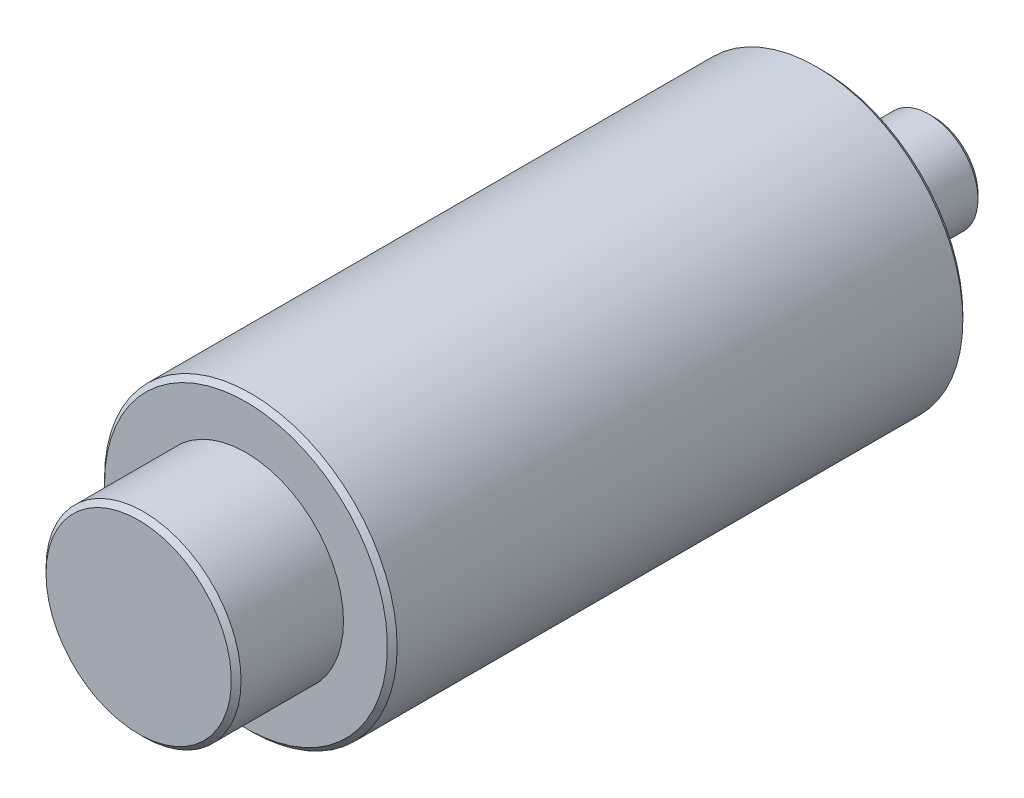
from build123d import *

# Parameters (mm, degrees)
CHAMFER1_SIZE = 0.5


with BuildPart() as part:
    # Sketch1 → Revolve1 (revolve)
    with BuildSketch(Plane(origin=(0, 0, 0), x_dir=(0, 0, -1), z_dir=(1, 0, 0)), mode=Mode.PRIVATE) as revolve1_sk:
        Polygon((81.5, 0), (81.5, 5.05), (73.5, 5.05), (73.5, 7.5), (70, 7.5), (70, 15), (11, 15), (11, 10), (0, 10), (0, 0), align=None)
    revolve(revolve1_sk.sketch.rotate(Axis((0, 0, 0), (0, 0, -1)), 90), axis=Axis((0, 0, 0), (0, 0, -1)))

    # Chamfer1
    chamfer1_edges = [part.edges().sort_by_distance(p)[0] for p in [
        (-7.5, 0, -73.5),
        (-5.05, 0, -81.5),
        (-10, 0, 0),
        (-15, 0, -11),
        (-15, 0, -70),
    ]]
    chamfer(chamfer1_edges, length=CHAMFER1_SIZE)


solid = part.part
